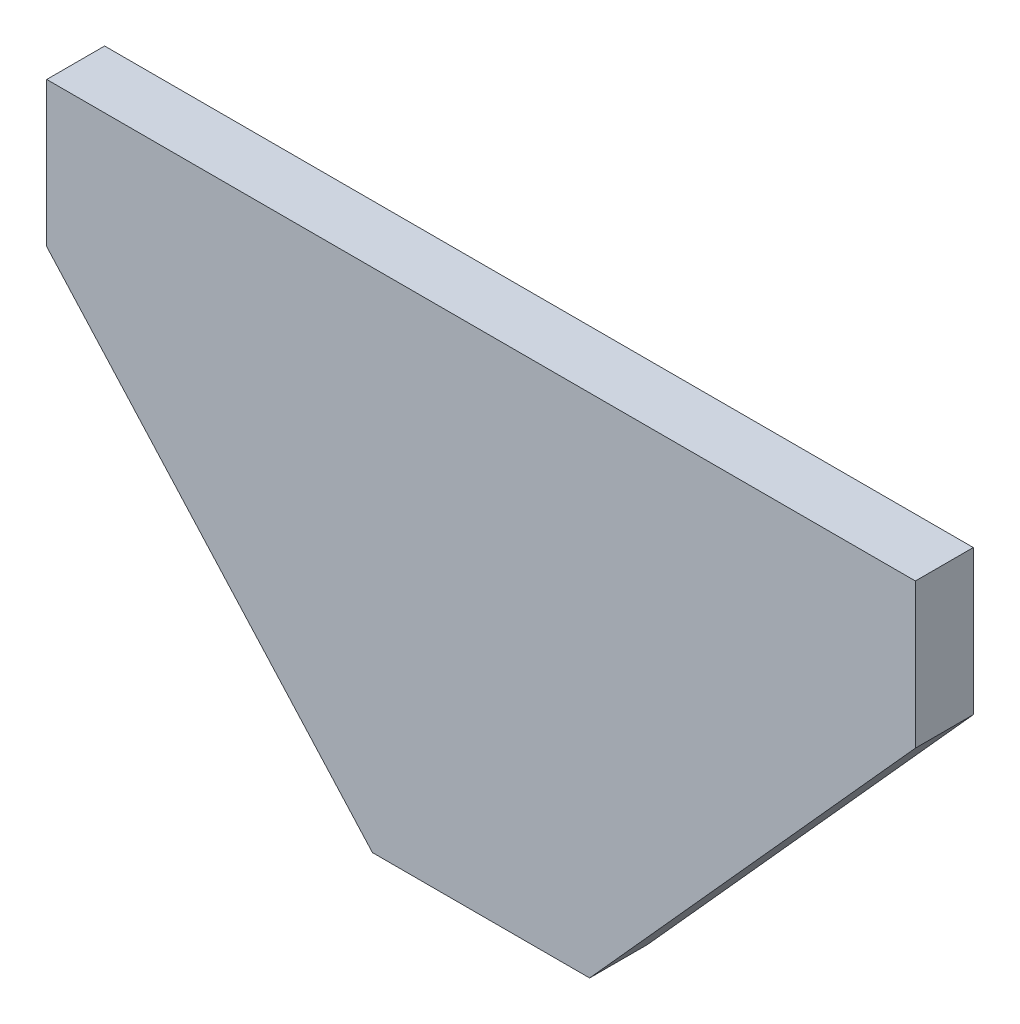
SolidWorks part; units mm, degrees
material "1023 碳钢板 (SS)"
ref_plane "Front Plane" through (0, 0, 0) normal (0, 0, 1) x (1, 0, 0)
ref_plane "Top Plane" through (0, 0, 0) normal (0, 1, 0) x (1, 0, 0)
ref_plane "Right Plane" through (0, 0, 0) normal (1, 0, 0) x (0, 0, -1)
sketch "Sketch1" plane through (0, 0, 0) normal (0, 0, 1) x (1, 0, 0)
  line L1 (-60, 35) -> (60, 35)
  line L2 (-60, 35) -> (-60, -35)
  line L3 (-60, -35) -> (60, -35)
  line L4 (60, 35) -> (60, -35)
  line L5 (-60, 35) -> (60, -35) construction
  line L6 (-60, -35) -> (60, 35) construction
  point P0 (0, 0)
  dimension "D1" = 120
  dimension "D2" = 70
extrude "Boss-Extrude1" add sketch "Sketch1" along normal blind 8
sketch "Sketch2" plane through (0, 0, 8) normal (0, 0, 1) x (1, 0, 0)
  line L0 (-60, 15) -> (-15, -35)
  line L2 (-60, -35) -> (60, -35) construction
  line L4 (15, -35) -> (60, 15)
  line L5 (60, -35) -> (60, 35) construction
  line L7 (-60, 15) -> (-60, -35)
  line L8 (-60, -35) -> (-15, -35)
  line L9 (60, 15) -> (60, -35)
  line L10 (60, -35) -> (15, -35)
  dimension "D1" = 50
  dimension "D2" = 45
  dimension "D3" = 50
extrude "Cut-Extrude1" cut sketch "Sketch2" against normal blind 8
